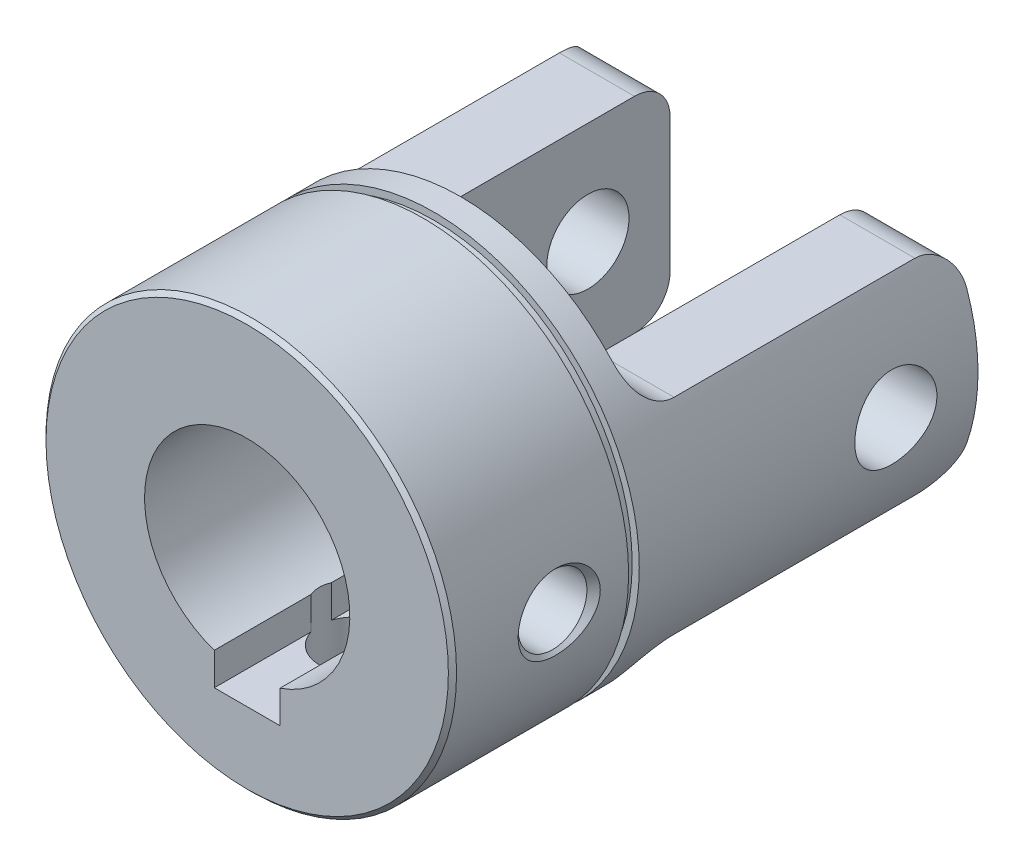
from build123d import *

# Parameters (mm, degrees)
CUT_EXTRUDE_1_DEPTH      = 25
CUT_EXTRUDE_1_DEPTH_BACK = 25
CUT_EXTRUDE_2_DEPTH      = 25
CUT_EXTRUDE_2_DEPTH_BACK = 25
SKETCH_3_W               = 25
SKETCH_3_H               = 38
CUT_EXTRUDE_3_DEPTH      = 25
CUT_EXTRUDE_3_DEPTH_BACK = 25
SKETCH_4_R               = 5
SKETCH_7_W               = 8
SKETCH_7_H               = 15.8
CUT_EXTRUDE_4_DEPTH      = 26


with BuildPart() as part:
    # 草图1 → 旋转1 (revolve)
    with BuildSketch(Plane(origin=(0, 0, 0), x_dir=(0, 0, -1), z_dir=(1, 0, 0)), mode=Mode.PRIVATE) as revolve_1_sk:
        Polygon((26, 0), (26, 12.5), (0, 12.5), (0, 24.5), (0.5, 25), (21.45, 25), (21.45, 24.133333333), (22.75, 24.133333333), (22.75, 25), (64, 25), (64, 0), align=None)
    revolve(revolve_1_sk.sketch.rotate(Axis((0, 0, -64), (0, 0, 1)), 270), axis=Axis((0, 0, -64), (0, 0, 1)))

    # 草图2 → 切除-拉伸1 (cut, two sides: drawn at the far end of the back side and taken through both)
    with BuildSketch(Plane(origin=(0, 0, 0), x_dir=(0, 0, -1), z_dir=(1, 0, 0)).offset(-CUT_EXTRUDE_1_DEPTH_BACK)):
        with BuildLine():
            Line((30.333333333, 12.5), (59.666666667, 12.5))
            ThreePointArc((59.666666667, 12.5), (62.730796052, 11.230796052), (64, 8.166666667))
            Line((64, 8.166666667), (64, -8.166666667))
            ThreePointArc((64, -8.166666667), (62.730796052, -11.230796052), (59.666666667, -12.5))
            Line((59.666666667, -12.5), (30.333333333, -12.5))
            ThreePointArc((30.333333333, -12.5), (27.269203948, -13.769203948), (26, -16.833333333))
            Line((26, -16.833333333), (26, -25))
            Line((26, -25), (69, -25))
            Line((69, -25), (69, 25))
            Line((69, 25), (26, 25))
            Line((26, 25), (26, 16.833333333))
            ThreePointArc((26, 16.833333333), (27.269203948, 13.769203948), (30.333333333, 12.5))
        make_face()
    extrude(amount=CUT_EXTRUDE_1_DEPTH + CUT_EXTRUDE_1_DEPTH_BACK, mode=Mode.SUBTRACT)

    # 草图3 → 切除-拉伸2 (cut, two sides: drawn at the far end of the back side and taken through both)
    with BuildSketch(Plane(origin=(0, 0, 0), x_dir=(1, 0, 0), z_dir=(0, 1, 0)).offset(-CUT_EXTRUDE_2_DEPTH_BACK)):
        with Locations((0, 45)):
            Rectangle(SKETCH_3_W, SKETCH_3_H)
    extrude(amount=CUT_EXTRUDE_2_DEPTH + CUT_EXTRUDE_2_DEPTH_BACK, mode=Mode.SUBTRACT)

    # 草图4 → 切除-拉伸3 (cut, two sides: drawn at the far end of the back side and taken through both)
    with BuildSketch(Plane(origin=(0, 0, 0), x_dir=(0, 0, -1), z_dir=(1, 0, 0)).offset(-CUT_EXTRUDE_3_DEPTH_BACK)):
        with Locations((54, 0)):
            Circle(SKETCH_4_R)
    extrude(amount=CUT_EXTRUDE_3_DEPTH + CUT_EXTRUDE_3_DEPTH_BACK, mode=Mode.SUBTRACT)

    # 草图5 → 切除-旋转1 (revolve, cut)
    with BuildSketch(Plane(origin=(0, 0, 0), x_dir=(0, 0, -1), z_dir=(1, 0, 0)), mode=Mode.PRIVATE) as cut_revolve_1_sk:
        Polygon((13, 0), (17.188, 0), (17.188, -24.188), (18, -25), (13, -25), align=None)
    revolve(cut_revolve_1_sk.sketch.rotate(Axis((0, -25, -13), (0, 1, 0)), 180), axis=Axis((0, -25, -13), (0, 1, 0)), mode=Mode.SUBTRACT)

    # 草图6 → 切除-旋转2 (revolve, cut)
    with BuildSketch(Plane(origin=(0, 0, 0), x_dir=(1, 0, 0), z_dir=(0, 1, 0)), mode=Mode.PRIVATE) as cut_revolve_2_sk:
        Polygon((25, 13), (25, 8), (24.188, 8.812), (0, 8.812), (0, 13), align=None)
    revolve(cut_revolve_2_sk.sketch.rotate(Axis((0, 0, -13), (1, 0, 0)), 180), axis=Axis((0, 0, -13), (1, 0, 0)), mode=Mode.SUBTRACT)

    # 草图7 → 切除-拉伸4 (cut)
    with BuildSketch(Plane.XY):
        with Locations((0, -7.9)):
            Rectangle(SKETCH_7_W, SKETCH_7_H)
    extrude(amount=-CUT_EXTRUDE_4_DEPTH, mode=Mode.SUBTRACT)


solid = part.part
